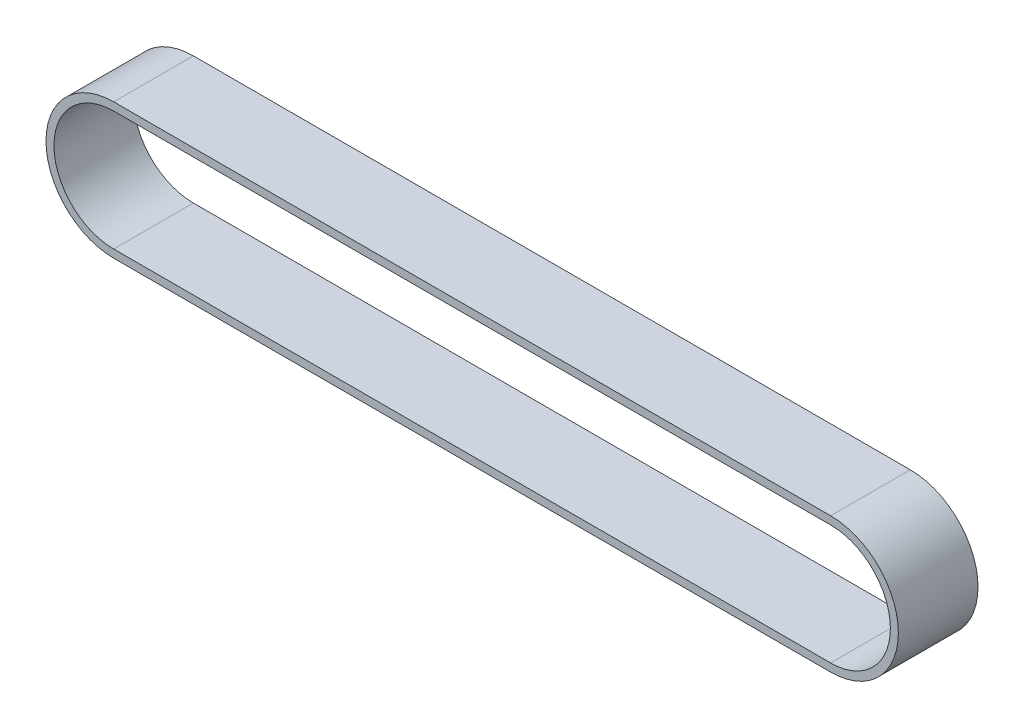
SolidWorks part; units mm, degrees
material "橡胶"
ref_plane "前视" through (0, 0, 0) normal (0, 0, 1) x (1, 0, 0)
ref_plane "上视" through (0, 0, 0) normal (0, 1, 0) x (1, 0, 0)
ref_plane "右视" through (0, 0, 0) normal (1, 0, 0) x (0, 0, -1)
sketch "草图1" plane through (0, 0, 0) normal (0, 0, 1) x (1, 0, 0)
  line L0 (-225, 0) -> (225, 0) construction
  line L1 (-225, 37.5) -> (225, 37.5)
  line L2 (-225, -37.5) -> (225, -37.5)
  line L3 (-225, 42.5) -> (225, 42.5)
  line L4 (-225, -42.5) -> (225, -42.5)
  arc A0 (-225, 37.5) -> (-225, -37.5) centre (-225, 0) ccw
  arc A1 (225, -37.5) -> (225, 37.5) centre (225, 0) ccw
  arc A2 (225, -42.5) -> (225, 42.5) centre (225, 0) ccw
  arc A3 (-225, 42.5) -> (-225, -42.5) centre (-225, 0) ccw
  point P2 (0, 0)
  dimension "D2" = 37.5
  dimension "D1" = 450
  dimension "D3" = 5
extrude "凸台-拉伸1" add sketch "草图1" along normal blind 50
